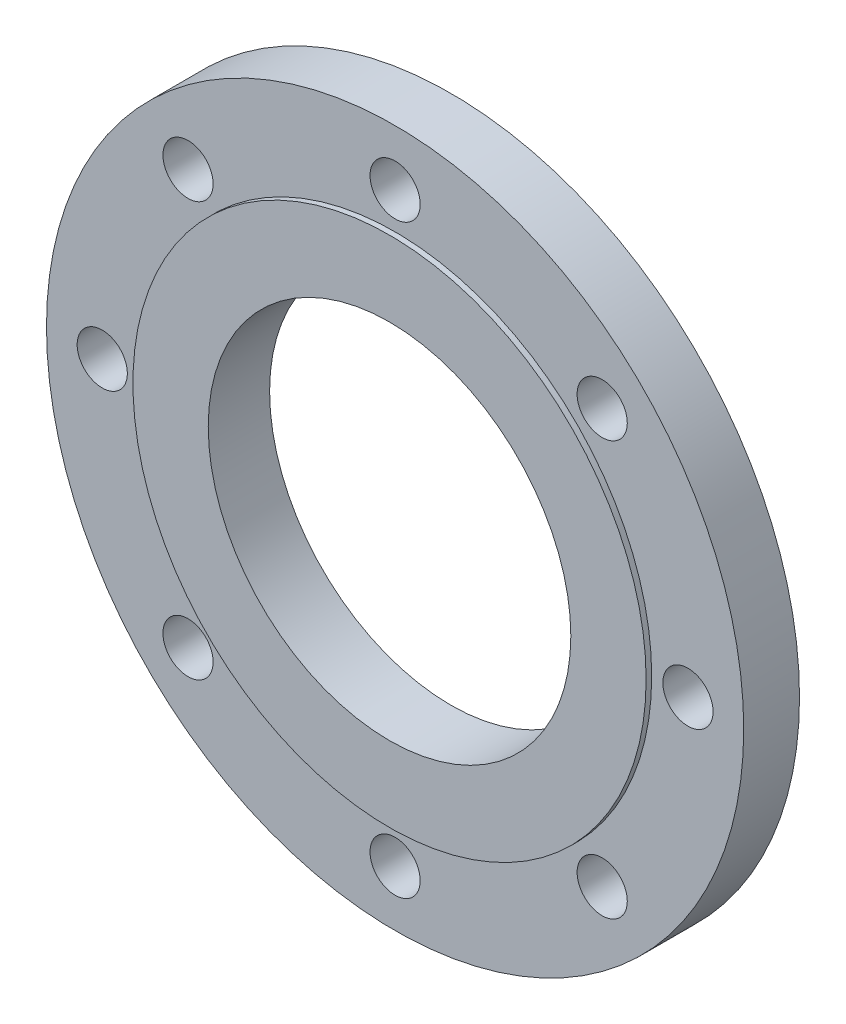
from build123d import *

# Parameters (mm, degrees)
SKETCH1_R           = 125
SKETCH1_R_2         = 65
SKETCH1_R_3         = 9
BOSS_EXTRUDE1_DEPTH = 20
SKETCH2_R           = 92
SKETCH2_R_2         = 65
BOSS_EXTRUDE2_DEPTH = 2


with BuildPart() as part:
    # Sketch1 → Boss-Extrude1 (new body)
    with BuildSketch(Plane.XY):
        Circle(SKETCH1_R)
        Circle(SKETCH1_R_2, mode=Mode.SUBTRACT)
        with Locations((0, 105)):
            Circle(SKETCH1_R_3, mode=Mode.SUBTRACT)
        with Locations((74.246212025, 74.246212025)):
            Circle(SKETCH1_R_3, mode=Mode.SUBTRACT)
        with Locations((105, 0)):
            Circle(SKETCH1_R_3, mode=Mode.SUBTRACT)
        with Locations((74.246212025, -74.246212025)):
            Circle(SKETCH1_R_3, mode=Mode.SUBTRACT)
        with Locations((0, -105)):
            Circle(SKETCH1_R_3, mode=Mode.SUBTRACT)
        with Locations((-74.246212025, -74.246212025)):
            Circle(SKETCH1_R_3, mode=Mode.SUBTRACT)
        with Locations((-105, 0)):
            Circle(SKETCH1_R_3, mode=Mode.SUBTRACT)
        with Locations((-74.246212025, 74.246212025)):
            Circle(SKETCH1_R_3, mode=Mode.SUBTRACT)
    extrude(amount=BOSS_EXTRUDE1_DEPTH)

    # Sketch2 → Boss-Extrude2 (add)
    with BuildSketch(Plane.XY.offset(20)):
        Circle(SKETCH2_R)
        Circle(SKETCH2_R_2, mode=Mode.SUBTRACT)
    extrude(amount=BOSS_EXTRUDE2_DEPTH)


solid = part.part
